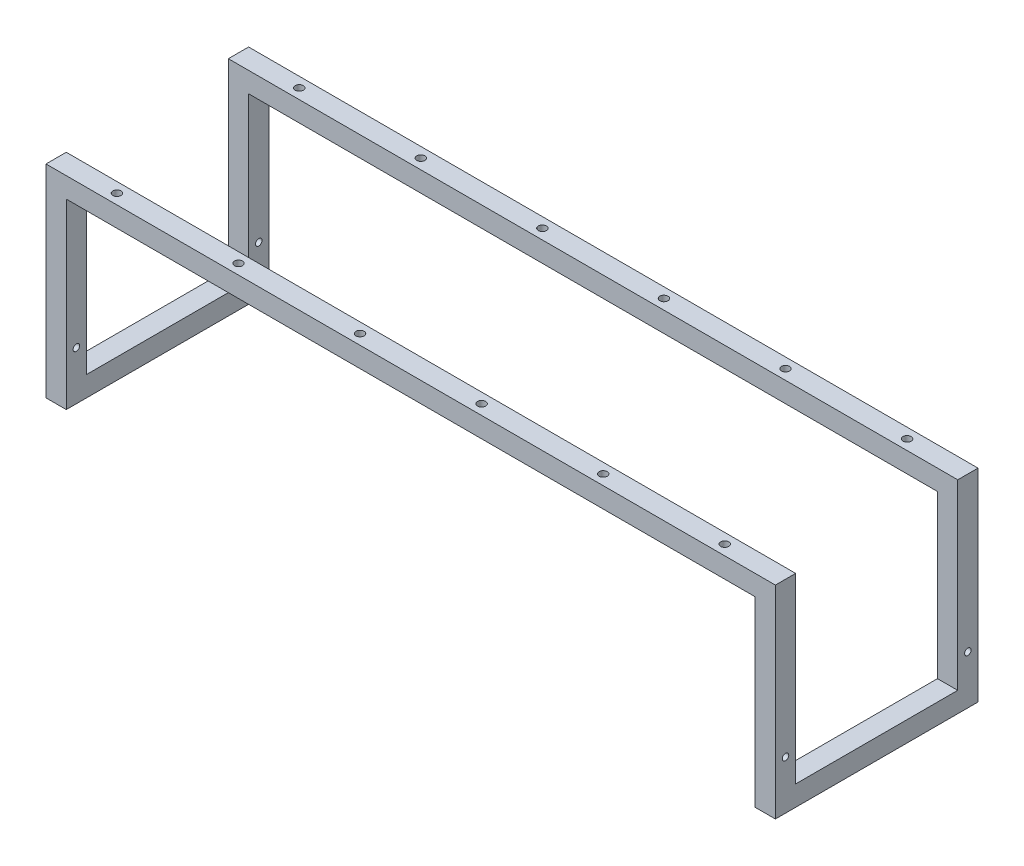
SolidWorks part; units mm, degrees
ref_plane "Front Plane" through (0, 0, 0) normal (0, 0, 1) x (1, 0, 0)
ref_plane "Top Plane" through (0, 0, 0) normal (0, 1, 0) x (1, 0, 0)
ref_plane "Right Plane" through (0, 0, 0) normal (1, 0, 0) x (0, 0, -1)
other "Configuration Table"
sketch "Sketch1" plane through (0, 0, 0) normal (0, 0, 1) x (1, 0, 0)
  line L1 (-25, -25) -> (25, -25)
  line L2 (-25, -25) -> (-25, 25)
  line L3 (-25, 25) -> (25, 25)
  line L4 (25, -25) -> (25, 25)
  line L5 (-25, -25) -> (25, 25) construction
  line L6 (-25, 25) -> (25, -25) construction
  point P0 (0, 0)
  dimension "D1" = 50
  dimension "D2" = 50
extrude "Boss-Extrude1" add sketch "Sketch1" along normal blind 500
sketch "Sketch2" plane through (0, 25, 0) normal (0, 1, 0) x (1, 0, 0)
  line L0 (25, -500) -> (25, 0) construction
  line L1 (-25, 0) -> (25, 0)
  line L2 (-25, 0) -> (-25, -50)
  line L3 (-25, -50) -> (25, -50)
  line L4 (25, 0) -> (25, -50)
  line L5 (-25, -500) -> (-25, 0) construction
  line L6 (25, -500) -> (-25, -500)
  line L7 (25, -500) -> (25, -450)
  line L8 (25, -450) -> (-25, -450)
  line L9 (-25, -500) -> (-25, -450)
  dimension "D1" = 50
  dimension "D2" = 50
extrude "Boss-Extrude2" add sketch "Sketch2" along normal blind 450
sketch "Sketch3" plane through (25, 0, 0) normal (1, 0, 0) x (0, 0, -1)
  line L0 (-450, 475) -> (-450, 25) construction
  line L1 (-500, 475) -> (-450, 475)
  line L2 (-500, 475) -> (-500, 425)
  line L3 (-500, 425) -> (-450, 425)
  line L4 (-450, 475) -> (-450, 425)
  line L5 (0, -25) -> (0, 475) construction
  line L6 (-50, 475) -> (0, 475)
  line L7 (-50, 475) -> (-50, 425)
  line L8 (-50, 425) -> (0, 425)
  line L9 (0, 475) -> (0, 425)
  dimension "D1" = 50
extrude "Boss-Extrude3" add sketch "Sketch3" along normal blind 1750
sketch "Sketch4" plane through (0, 425, 0) normal (0, -1, 0) x (-1, 0, 0)
  line L0 (-1775, -450) -> (-25, -450) construction
  line L1 (-1775, -500) -> (-1725, -500)
  line L2 (-1775, -500) -> (-1775, -450)
  line L3 (-1775, -450) -> (-1725, -450)
  line L4 (-1725, -500) -> (-1725, -450)
  line L5 (-1775, -50) -> (-25, -50) construction
  line L6 (-1775, 0) -> (-1725, 0)
  line L7 (-1775, 0) -> (-1775, -50)
  line L8 (-1775, -50) -> (-1725, -50)
  line L9 (-1725, 0) -> (-1725, -50)
  dimension "D1" = 50
extrude "Boss-Extrude4" add sketch "Sketch4" along normal blind 450
sketch "Sketch5" plane through (0, 0, 450) normal (0, 0, -1) x (-1, 0, 0)
  line L0 (-1775, -25) -> (-1775, 475) construction
  line L1 (-1725, -25) -> (-1775, -25)
  line L2 (-1725, -25) -> (-1725, 25)
  line L3 (-1725, 25) -> (-1775, 25)
  line L4 (-1775, -25) -> (-1775, 25)
  dimension "D1" = 50
extrude "Boss-Extrude5" add sketch "Sketch5" along normal blind 400
sketch "Sketch6" plane through (0, 475, 0) normal (0, 1, 0) x (1, 0, 0)
  line L0 (-25, -25) -> (1775, -25) construction
  line L1 (-25, 0) -> (-25, -50) construction
  line L2 (1775, 0) -> (1775, -50) construction
  line L3 (-25, -475) -> (1775, -475) construction
  line L4 (-25, -450) -> (-25, -500) construction
  line L5 (1775, -450) -> (1775, -500) construction
  line L6 (125, -25) -> (125, -475) construction
  circle A0 centre (125, -25) radius 10
  circle A1 centre (125, -475) radius 10
  dimension "D2" = 20
  dimension "D1" = 150
extrude "Cut-Extrude1" cut sketch "Sketch6" against normal up to next
pattern_linear "LPattern1" count 6 spacing 300 along (1, 0, 0) of "Cut-Extrude1"
sketch "Sketch8" plane through (-25, 0, 0) normal (-1, 0, 0) x (0, 0, 1)
  line L0 (0, 95) -> (500, 95) construction
  line L1 (0, 475) -> (0, -25) construction
  line L2 (500, 475) -> (500, -25) construction
  line L3 (500, -25) -> (0, -25) construction
  line L4 (25, 475) -> (25, -25) construction
  line L5 (0, 475) -> (50, 475) construction
  line L6 (475, 475) -> (475, -25) construction
  line L7 (450, 475) -> (500, 475) construction
  circle A0 centre (475, 95) radius 8
  circle A1 centre (25, 95) radius 8
  dimension "D2" = 16
  dimension "D1" = 120
extrude "Cut-Extrude2" cut sketch "Sketch8" against normal through all
sketch "Sketch9" plane through (0, 0, 450) normal (0, 0, -1) x (-1, 0, 0)
  line L0 (25, 475) -> (25, 25) construction
  line L1 (10, 115) -> (25, 115)
  line L2 (10, 115) -> (10, 75)
  line L3 (10, 75) -> (25, 75)
  line L4 (25, 115) -> (25, 75)
  line L5 (10, 115) -> (25, 75) construction
  line L6 (10, 75) -> (25, 115) construction
  line L7 (25, -25) -> (-25, -25) construction
  point P0 (17.5, 95)
  dimension "D1" = 15
  dimension "D2" = 40
  dimension "D3" = 100
extrude "Boss-Extrude6" add sketch "Sketch9" along normal blind 30
sketch "Sketch12" plane through (0, 0, 0) normal (0, 0, -1) x (-1, 0, 0)
  line L0 (25, 475) -> (25, -25) construction
  line L1 (25, 115) -> (10, 115)
  line L2 (25, 115) -> (25, 75)
  line L3 (25, 75) -> (10, 75)
  line L4 (10, 115) -> (10, 75)
  line L7 (25, -25) -> (-25, -25) construction
  dimension "D1" = 15
  dimension "D2" = 40
  dimension "D3" = 100
extrude "Boss-Extrude7" add sketch "Sketch12" along normal blind 30
sketch "Sketch13" plane through (-25, 0, 0) normal (-1, 0, 0) x (0, 0, 1)
  line L0 (-30, 75) -> (0, 75) construction
  line L1 (-30, 115) -> (-15, 115)
  line L2 (-30, 115) -> (-30, 75)
  line L3 (-30, 75) -> (-15, 75)
  line L4 (-15, 115) -> (-15, 75)
  line L5 (420, 75) -> (450, 75) construction
  line L6 (420, 115) -> (435, 115)
  line L7 (420, 115) -> (420, 75)
  line L8 (420, 75) -> (435, 75)
  line L9 (435, 115) -> (435, 75)
  dimension "D1" = 15
  dimension "D2" = 15
extrude "Boss-Extrude8" add sketch "Sketch13" along normal blind 48
sketch "Sketch14" plane through (0, 0, -30) normal (0, 0, -1) x (-1, 0, 0)
  line L0 (73, 115) -> (73, 75) construction
  circle A0 centre (53, 95) radius 7.5
  dimension "D1" = 15
  dimension "D2" = 20
extrude "Cut-Extrude3" cut sketch "Sketch14" against normal through all both and the other way through all
sketch "Sketch15" plane through (0, 0, -30) normal (0, 0, -1) x (-1, 0, 0)
  circle A0 centre (53, 95) radius 7.5
  circle A1 centre (53, 95) radius 5.5
  dimension "D1" = 11
extrude "Boss-Extrude9" add sketch "Sketch15" against normal blind 15
